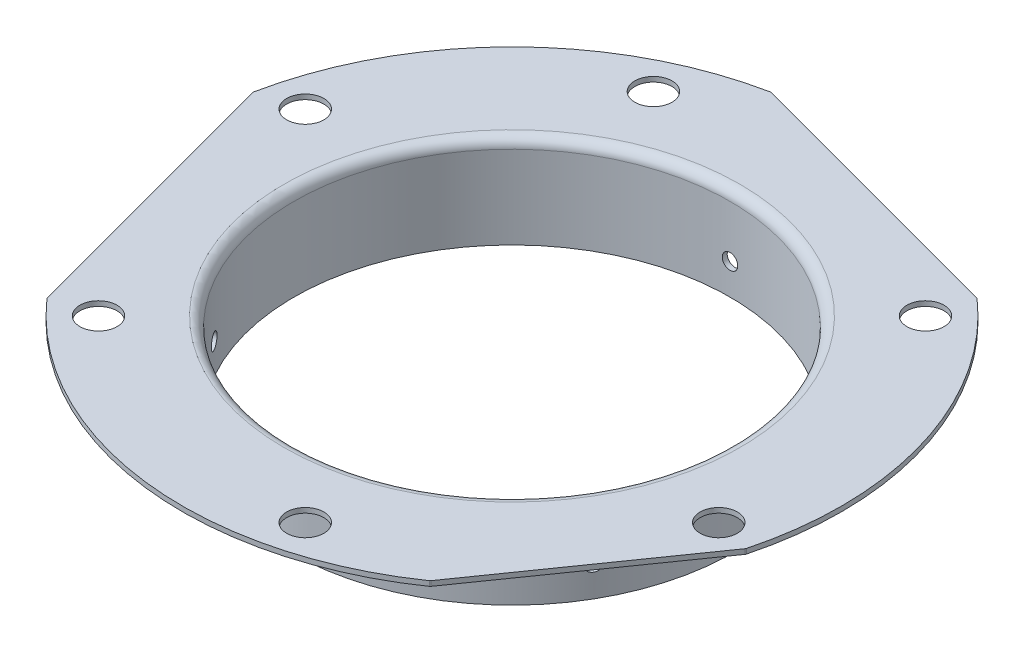
SolidWorks part; units mm, degrees
material "SPHC"
ref_plane "Front Plane" through (0, 0, 0) normal (0, 0, 1) x (1, 0, 0)
ref_plane "Top Plane" through (0, 0, 0) normal (0, 1, 0) x (1, 0, 0)
ref_plane "Right Plane" through (0, 0, 0) normal (1, 0, 0) x (0, 0, -1)
sketch "Sketch1" plane through (0, 0, 0) normal (1, 0, 0) x (0, 0, -1)
  line L0 (0, 0) -> (0, -26.8) construction
  line L1 (-106.5, 0) -> (-73.7, 0)
  line L2 (-70.5, -3.2) -> (-70.5, -30)
  line L3 (-106.5, -1.6) -> (-73.7, -1.6)
  line L4 (-72.1, -3.2) -> (-72.1, -30)
  line L5 (-106.5, 0) -> (-106.5, -1.6)
  line L6 (-72.1, -30) -> (-70.5, -30)
  arc A0 (-73.7, 0) -> (-70.5, -3.2) centre (-73.7, -3.2) cw
  arc A1 (-73.7, -1.6) -> (-72.1, -3.2) centre (-73.7, -3.2) cw
  point P9 (-70.5, 0)
  dimension "D4" = 3.2
  dimension "D1" = 213
  dimension "D2" = 141
  dimension "D3" = 30
  dimension "D5" = 1.6
revolve "Revolve1" add sketch "Sketch1" angle 360 about L0
sketch "Sketch2" plane through (0, 0, 0) normal (0, 1, 0) x (1, 0, 0)
  line L0 (0, 0) -> (-106.5, 0) construction
  line L1 (0, 0) -> (0, -106.5) construction
  line L2 (0, 0) -> (-91.28, 24.4584) construction
  line L3 (0, 0) -> (-39.9374, 85.6461) construction
  line L4 (0, 0) -> (66.8216, 66.8216) construction
  line L5 (0, 0) -> (91.28, -24.4584) construction
  line L6 (0, 0) -> (24.4584, -91.28) construction
  line L7 (0, 0) -> (-66.8216, -66.8216) construction
  circle A16 centre (0, 0) radius 106.5 construction
  circle A17 centre (0, 0) radius 94.5 construction
  circle A18 centre (-91.28, 24.4584) radius 6
  circle A19 centre (-39.9374, 85.6461) radius 6
  circle A20 centre (66.8216, 66.8216) radius 6
  circle A21 centre (91.28, -24.4584) radius 6
  circle A22 centre (24.4584, -91.28) radius 6
  circle A23 centre (-66.8216, -66.8216) radius 6
  dimension "D1" = 189
  dimension "D8" = 60
  dimension "D9" = 45
  dimension "D3" = 12
  dimension "D2" = 15
  dimension "D4" = 50
  dimension "D5" = 70
  dimension "D6" = 60
  dimension "D7" = 60
extrude "Cut-Extrude1" cut sketch "Sketch2" against normal up to next
sketch "Sketch3" plane through (0, 0, 0) normal (0, 1, 0) x (1, 0, 0)
  line L0 (0, 0) -> (24.4584, -91.28) construction
  line L1 (-80.0457, -70.2491) -> (-104.4462, 20.8147)
  line L2 (0, 0) -> (-91.28, 24.4584) construction
  line L3 (-20.8147, 104.4462) -> (70.2491, 80.0457)
  line L4 (0, 0) -> (61.0859, 87.2397) construction
  line L5 (60.9012, -87.3687) -> (102.9292, -27.3466)
  circle A0 centre (0, 0) radius 106.5 construction
  arc A1 (60.9012, -87.3687) -> (102.9292, -27.3466) centre (0, 0) ccw
  arc A2 (-104.4462, 20.8147) -> (-80.0457, -70.2491) centre (0, 0) ccw
  arc A3 (70.2491, 80.0457) -> (-20.8147, 104.4462) centre (0, 0) ccw
  dimension "D1" = 95.5
  dimension "D2" = 95.5
  dimension "D3" = 70
  dimension "D4" = 100
extrude "Cut-Extrude2" cut sketch "Sketch3" against normal up to next
fillet "Fillet1" radius 1 6 edges at (102.9292, -0.8, 27.3466) (60.9012, -0.8, 87.3687) (-80.0457, -0.8, 70.2491) (-104.4462, -0.8, -20.8147) (-20.8147, -0.8, -104.4462) (70.2491, -0.8, -80.0457)
sketch "Sketch4" plane through (0, 0, 0) normal (0, 0, 1) x (1, 0, 0)
  line L0 (-70.5, -30) -> (70.5, -30) construction
  circle A0 centre (0, -20) radius 2.5
  dimension "D1" = 5
  dimension "D2" = 10
extrude "Cut-Extrude3" cut sketch "Sketch4" against normal up to next
pattern_circular "CirPattern1" count 3 over 360 about axis through (0, -30, 0) along (0, 1, 0) of "Cut-Extrude3"
